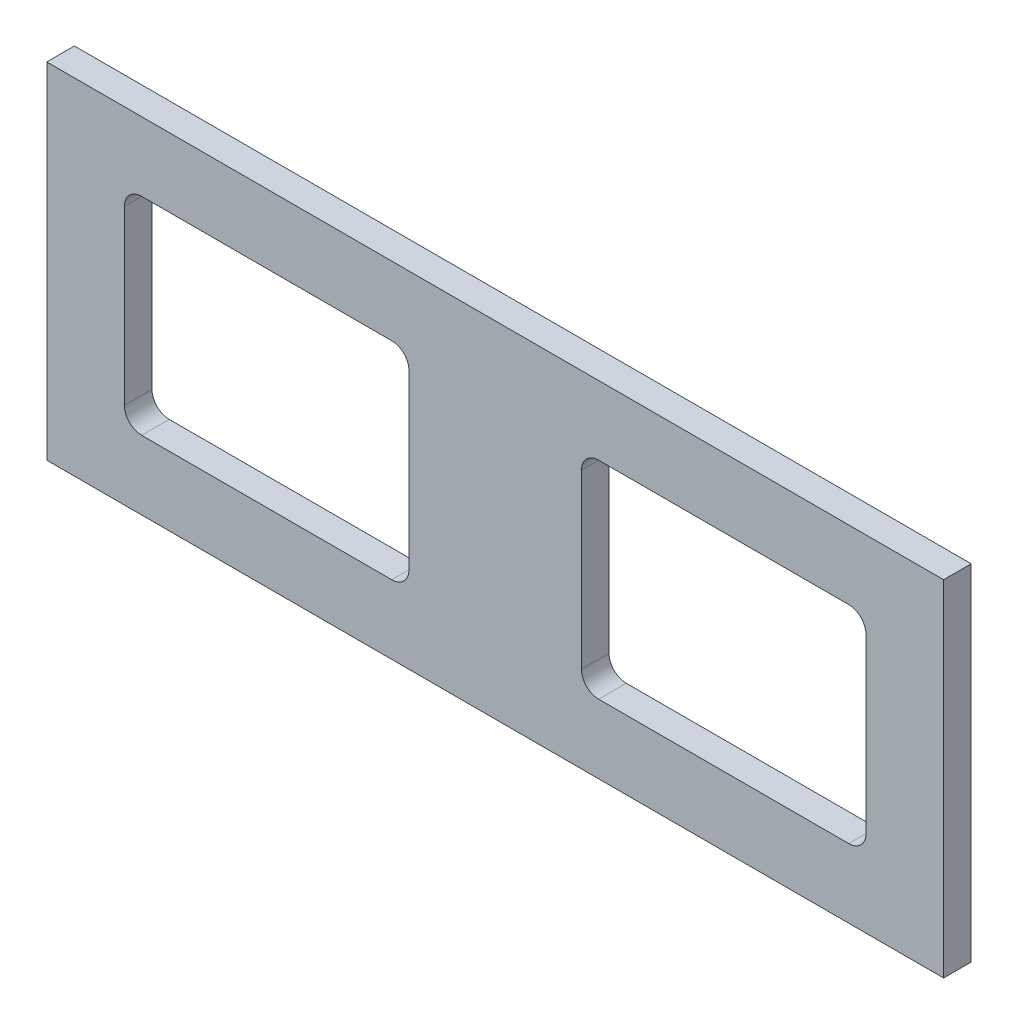
from build123d import *

# Parameters (mm, degrees)
SKETCH1_W           = 520
SKETCH1_H           = 200
BOSS_EXTRUDE1_DEPTH = 16


with BuildPart() as part:
    # Sketch1 → Boss-Extrude1 (new body)
    with BuildSketch(Plane.XY):
        with Locations((154.849239326, 69.96508599)):
            Rectangle(SKETCH1_W, SKETCH1_H)
        with BuildLine():
            Line((345.350111085, 9.96508599), (214.849239326, 9.96508599))
            ThreePointArc((214.849239326, 9.96508599), (207.778171514, 12.894018179), (204.849239326, 19.96508599))
            Line((204.849239326, 19.96508599), (204.849239326, 119.96508599))
            ThreePointArc((204.849239326, 119.96508599), (207.778171514, 127.036153802), (214.849239326, 129.96508599))
            Line((214.849239326, 129.96508599), (359.849239326, 129.96508599))
            ThreePointArc((359.849239326, 129.96508599), (366.920307138, 127.036153802), (369.849239326, 119.96508599))
            Line((369.849239326, 119.96508599), (369.849239326, 19.96508599))
            ThreePointArc((369.849239326, 19.96508599), (366.920307138, 12.894018179), (359.849239326, 9.96508599))
            Line((359.849239326, 9.96508599), (345.350111085, 9.96508599))
        make_face(mode=Mode.SUBTRACT)
        with BuildLine():
            Line((104.849239326, 19.96508599), (104.849239326, 119.96508599))
            ThreePointArc((104.849239326, 119.96508599), (101.920307138, 127.036153802), (94.849239326, 129.96508599))
            Line((94.849239326, 129.96508599), (-50.150760674, 129.96508599))
            ThreePointArc((-50.150760674, 129.96508599), (-57.221828486, 127.036153802), (-60.150760674, 119.96508599))
            Line((-60.150760674, 119.96508599), (-60.150760674, 19.96508599))
            ThreePointArc((-60.150760674, 19.96508599), (-57.221828486, 12.894018179), (-50.150760674, 9.96508599))
            Line((-50.150760674, 9.96508599), (-35.651632433, 9.96508599))
            Line((-35.651632433, 9.96508599), (94.849239326, 9.96508599))
            ThreePointArc((94.849239326, 9.96508599), (101.920307138, 12.894018179), (104.849239326, 19.96508599))
        make_face(mode=Mode.SUBTRACT)
    extrude(amount=BOSS_EXTRUDE1_DEPTH)


solid = part.part
